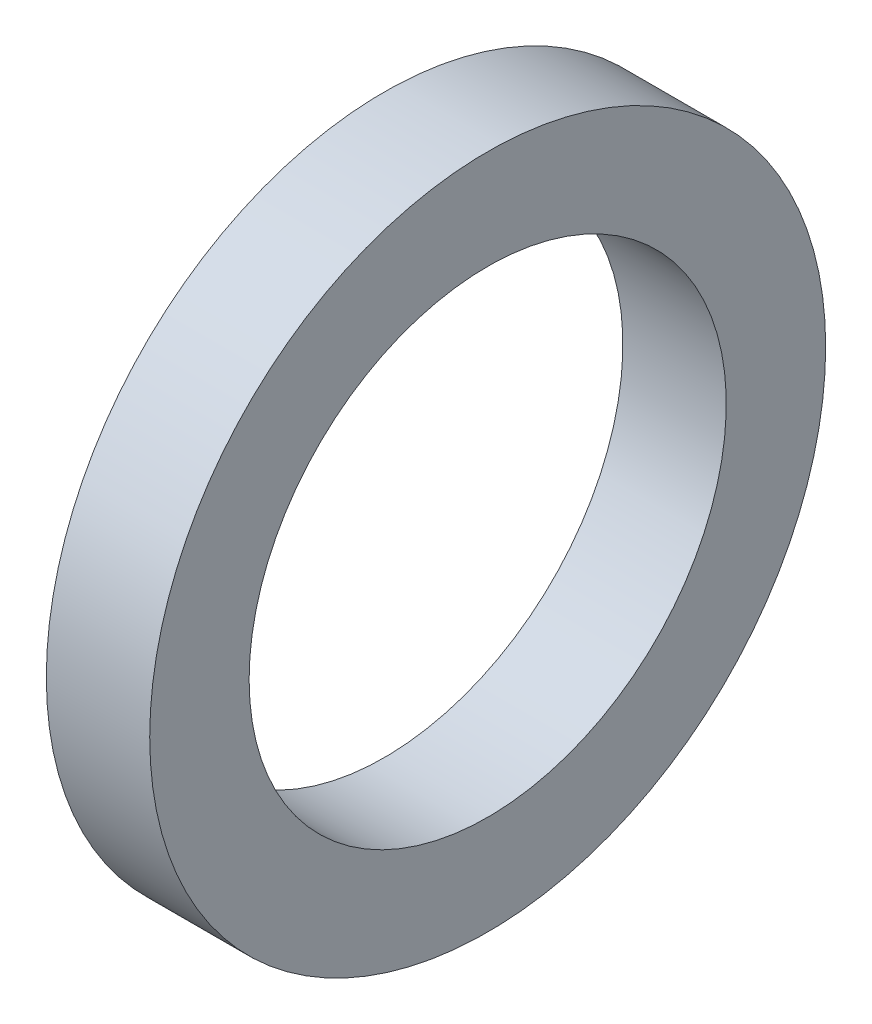
SolidWorks part; units mm, degrees
ref_plane "前视" through (0, 0, 0) normal (0, 0, 1) x (1, 0, 0)
ref_plane "上视" through (0, 0, 0) normal (0, 1, 0) x (1, 0, 0)
ref_plane "右视" through (0, 0, 0) normal (1, 0, 0) x (0, 0, -1)
sketch "草图1" plane through (0, 0, 0) normal (1, 0, 0) x (0, 0, -1)
  circle A0 centre (0, 0) radius 42.5
  circle A1 centre (0, 0) radius 30
  dimension "D1" = 60
  dimension "D2" = 85
extrude "凸台-拉伸1" add sketch "草图1" along normal blind 13
